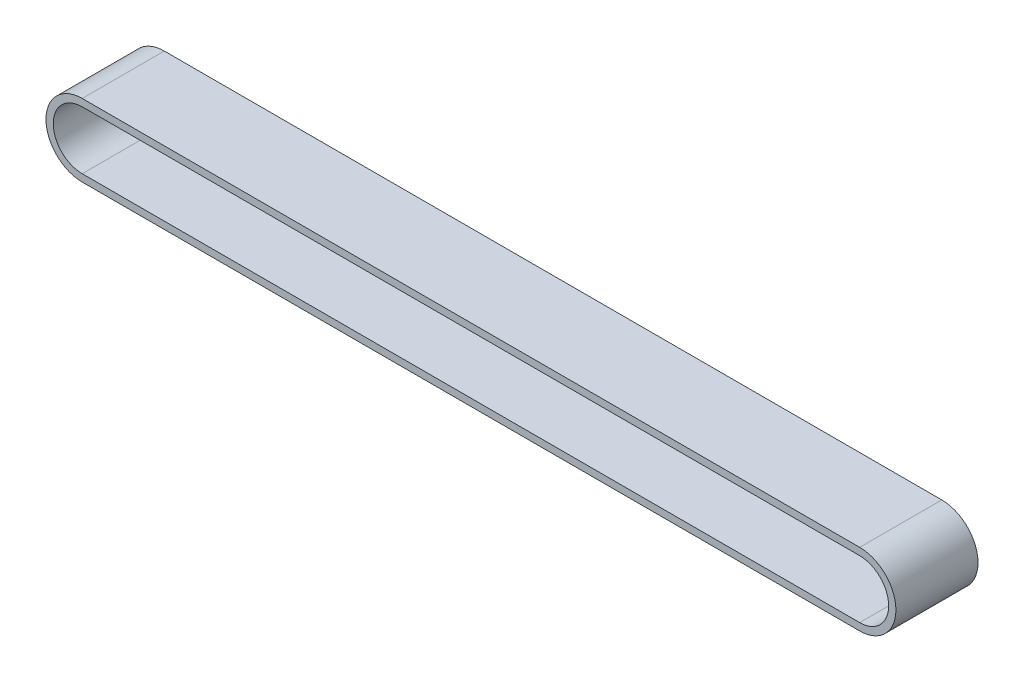
from build123d import *

# Parameters (mm, degrees)
EXTRUDE_1_DEPTH = 170


with BuildPart() as part:
    # 草图1 → 凸台-拉伸1 (new body)
    with BuildSketch(Plane.XY):
        with BuildLine():
            Line((0, 75), (-1610, 75))
            ThreePointArc((-1610, 75), (-1685, 0), (-1610, -75))
            Line((-1610, -75), (0, -75))
            ThreePointArc((0, -75), (75, 0), (0, 75))
        make_face()
        with BuildLine():
            Line((0, 60), (-1610, 60))
            ThreePointArc((-1610, 60), (-1670, 0), (-1610, -60))
            Line((-1610, -60), (0, -60))
            ThreePointArc((0, -60), (60, 0), (0, 60))
        make_face(mode=Mode.SUBTRACT)
    extrude(amount=EXTRUDE_1_DEPTH)


solid = part.part
